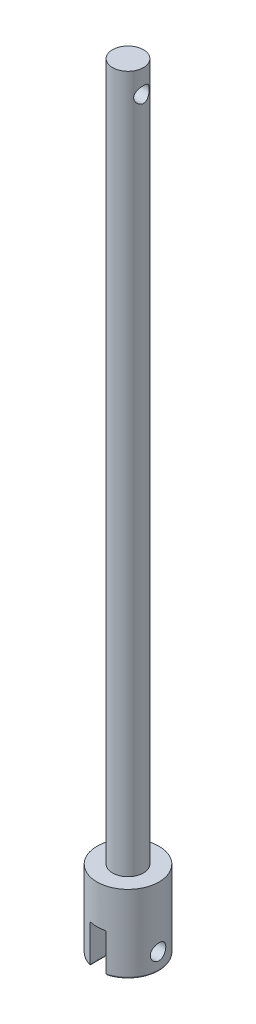
from build123d import *

# Parameters (mm, degrees)
SKETCH_11_R         = 2
EXTRUDE_3_DEPTH     = 100
SKETCH_20_R         = 4
EXTRUDE_4_DEPTH     = 10
SKETCH_16_W         = 2.1
SKETCH_16_H         = 5
CUT_EXTRUDE_5_DEPTH = 200
SKETCH_18_R         = 1
CUT_EXTRUDE_7_DEPTH = 200
SKETCH_19_R         = 1
CUT_EXTRUDE_8_DEPTH = 5
FILLET_1_R          = 0.2
FILLET_2_R          = 0.2


with BuildPart() as part:
    # 草图11 → 凸台-拉伸3 (new body)
    with BuildSketch(Plane.XZ):
        with Locations(Location((0, 0, 0), (0, 0, 270))):
            Circle(SKETCH_11_R)
    extrude(amount=EXTRUDE_3_DEPTH)

    # 草图20 → 凸台-拉伸4 (add)
    with BuildSketch(Plane.XZ.offset(100)):
        with Locations(Location((0, 0, 0), (0, 0, 270))):
            Circle(SKETCH_20_R)
    extrude(amount=-EXTRUDE_4_DEPTH)

    # 草图16 → 切除-拉伸5 (cut, symmetric)
    with BuildSketch(Plane.XY):
        with Locations((0, -97.5)):
            Rectangle(SKETCH_16_W, SKETCH_16_H)
    extrude(amount=CUT_EXTRUDE_5_DEPTH, both=True, mode=Mode.SUBTRACT)

    # 草图18 → 切除-拉伸7 (cut, symmetric)
    with BuildSketch(Plane(origin=(-1.05, 0, 0), x_dir=(0, 0, -1), z_dir=(1, 0, 0))):
        with Locations(Location((0, -97.8, 0), (0, 0, 90))):
            Circle(SKETCH_18_R)
    extrude(amount=CUT_EXTRUDE_7_DEPTH, both=True, mode=Mode.SUBTRACT)

    # 草图19 → 切除-拉伸8 (cut, symmetric)
    with BuildSketch(Plane(origin=(0, 0, 0), x_dir=(0, 0, -1), z_dir=(1, 0, 0))):
        with Locations((0, -3)):
            Circle(SKETCH_19_R)
    extrude(amount=CUT_EXTRUDE_8_DEPTH, both=True, mode=Mode.SUBTRACT)

    # 圆角1
    fillet_1_edges = [part.edges().sort_by_distance(p)[0] for p in [
        (-4, -100, 0),
        (1.05, -100, 0),
        (-1.05, -100, 0),
        (4, -100, 0),
    ]]
    fillet(fillet_1_edges, radius=FILLET_1_R)

    # 圆角2
    fillet_2_edges = [part.edges().sort_by_distance(p)[0] for p in [
        (-1.05, -95, 0),
        (1.05, -95, 0),
    ]]
    fillet(fillet_2_edges, radius=FILLET_2_R)


solid = part.part
